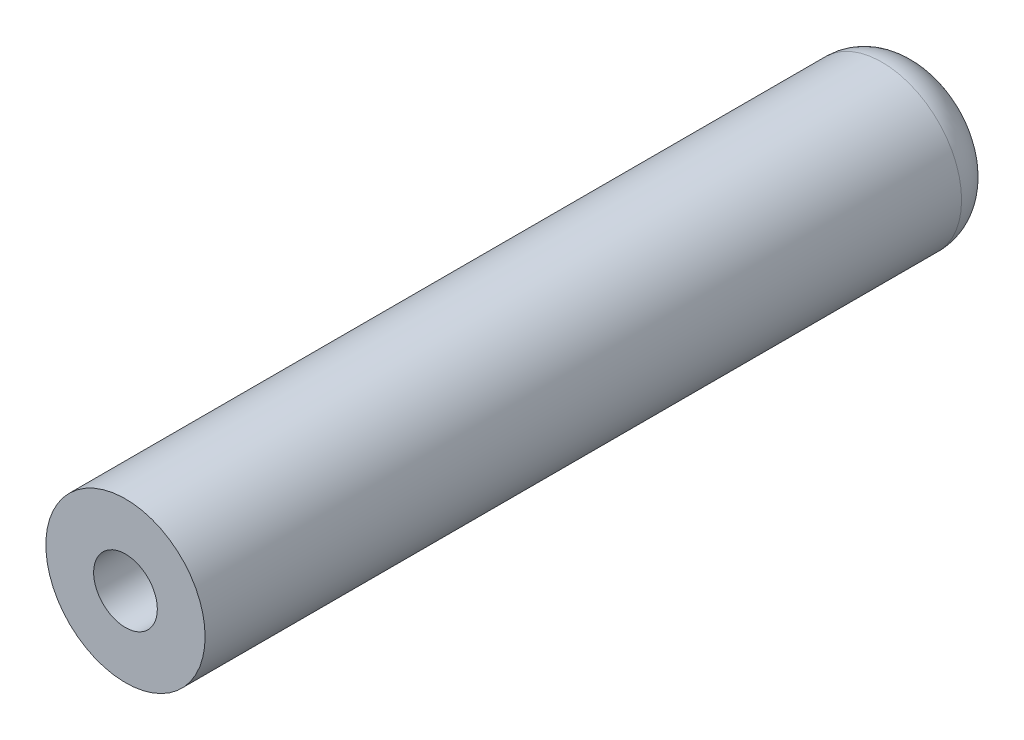
from build123d import *

# Parameters (mm, degrees)
SKETCH1_R             = 2
BOSS_EXTRUDE1_DEPTH   = 20
M2_TAPPED_HOLE1_D     = 1.6
M2_TAPPED_HOLE1_DEPTH = 5.2
M2_TAPPED_HOLE1_TIP   = 0.480688495
FILLET1_R             = 1


with BuildPart() as part:
    # Sketch1 → Boss-Extrude1 (new body)
    with BuildSketch(Plane.XY):
        with Locations((10.281246694, -38.2)):
            Circle(SKETCH1_R)
    extrude(amount=BOSS_EXTRUDE1_DEPTH)

    # M2 Tapped Hole1
    with Locations(Plane(origin=(10.281246694, -38.2, 23.7), x_dir=(0, 1, 0), z_dir=(0, 0, 1))):
        with Locations((0, 0)):
            Hole(M2_TAPPED_HOLE1_D / 2, depth=M2_TAPPED_HOLE1_DEPTH)
            with Locations((0, 0, -(M2_TAPPED_HOLE1_DEPTH + M2_TAPPED_HOLE1_TIP / 2))):  # 118° drill point
                Cone(0, M2_TAPPED_HOLE1_D / 2, M2_TAPPED_HOLE1_TIP, mode=Mode.SUBTRACT)

    # Fillet1
    fillet1_edges = [part.edges().sort_by_distance(p)[0] for p in [
        (8.281246694, -38.2, 0),
    ]]
    fillet(fillet1_edges, radius=FILLET1_R)


solid = part.part
